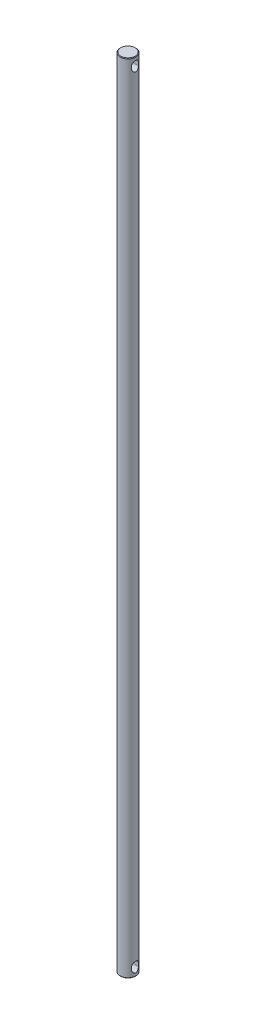
from build123d import *

# Parameters (mm, degrees)
SKETCH_1_R               = 7
EXTRUDE_1_DEPTH          = 357.5
CHAMFER_1_SIZE           = 0.5
CUT_EXTRUDE_1_DEPTH      = 358.637036673
CUT_EXTRUDE_1_DEPTH_BACK = 358.637036673


with BuildPart() as part:
    # 草图1 → 凸台-拉伸1 (new, symmetric)
    with BuildSketch(Plane(origin=(0, 0, 0), x_dir=(1, 0, 0), z_dir=(0, 1, 0))):
        with Locations(Location((0, 0, 0), (0, 0, 270))):
            Circle(SKETCH_1_R)
    extrude(amount=EXTRUDE_1_DEPTH, both=True)

    # 倒角1
    chamfer_1_edges = [part.edges().sort_by_distance(p)[0] for p in [
        (0, -357.5, -7),
        (0, 357.5, -7),
    ]]
    chamfer(chamfer_1_edges, length=CHAMFER_1_SIZE)

    # 草图2 → 切除-拉伸1 (cut, two sides: drawn at the far end of the back side and taken through both)
    with BuildSketch(Plane(origin=(0, 0, 0), x_dir=(0, 0, -1), z_dir=(1, 0, 0)).offset(-CUT_EXTRUDE_1_DEPTH_BACK)):
        with BuildLine():
            Line((-3, -351.5), (-3, -348.5))
            ThreePointArc((-3, -348.5), (0, -345.5), (3, -348.5))
            Line((3, -348.5), (3, -351.5))
            ThreePointArc((3, -351.5), (0, -354.5), (-3, -351.5))
        make_face()
        with BuildLine():
            Line((-3, 351.5), (-3, 348.5))
            ThreePointArc((-3, 348.5), (0, 345.5), (3, 348.5))
            Line((3, 348.5), (3, 351.5))
            ThreePointArc((3, 351.5), (0, 354.5), (-3, 351.5))
        make_face()
    extrude(amount=CUT_EXTRUDE_1_DEPTH + CUT_EXTRUDE_1_DEPTH_BACK, mode=Mode.SUBTRACT)


solid = part.part
